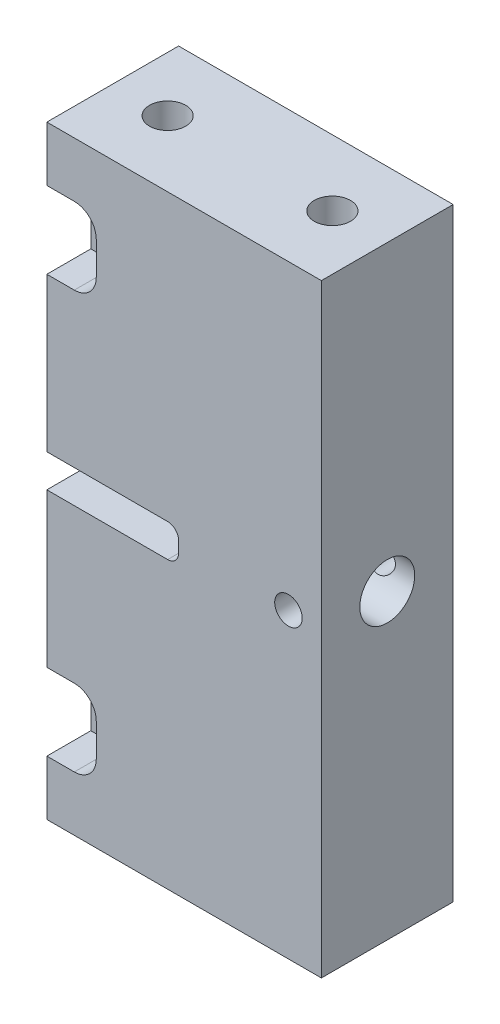
SolidWorks part; units mm, degrees
material "6061铝"
ref_plane "前视基准面" through (0, 0, 0) normal (0, 0, 1) x (1, 0, 0)
ref_plane "上视基准面" through (0, 0, 0) normal (0, 1, 0) x (1, 0, 0)
ref_plane "右视基准面" through (0, 0, 0) normal (1, 0, 0) x (0, 0, -1)
sketch "草图1" plane through (0, 0, 0) normal (1, 0, 0) x (0, 0, -1)
  line L1 (-6, 27.5) -> (6, 27.5)
  line L2 (-6, 27.5) -> (-6, -27.5)
  line L3 (-6, -27.5) -> (6, -27.5)
  line L4 (6, 27.5) -> (6, -27.5)
  line L5 (-6, 27.5) -> (6, -27.5) construction
  line L6 (-6, -27.5) -> (6, 27.5) construction
  point P0 (0, 0)
  dimension "D1" = 12
  dimension "D2" = 55
extrude "凸台-拉伸1" add sketch "草图1" along normal blind 25
sketch "草图2" plane through (25, 0, 0) normal (1, 0, 0) x (0, 0, -1)
  circle A0 centre (0, 0) radius 1.1
  dimension "D1" = 2.2
extrude "切除-拉伸1" cut sketch "草图2" against normal blind 25
sketch "草图3" plane through (25, 0, 0) normal (1, 0, 0) x (0, 0, -1)
  circle A0 centre (0, 0) radius 2.5
  dimension "D1" = 5
extrude "切除-拉伸2" cut sketch "草图3" against normal blind 8
chamfer "倒角1" [suppressed] distance 1 angle 45
sketch "草图4" plane through (0, 0, 6) normal (0, 0, 1) x (1, 0, 0)
  line L0 (0, 27.5) -> (0, -27.5) construction
  line L1 (-12, 1.5) -> (12, 1.5)
  line L2 (-12, 1.5) -> (-12, -1.5)
  line L3 (-12, -1.5) -> (12, -1.5)
  line L4 (12, 1.5) -> (12, -1.5)
  line L5 (-12, 1.5) -> (12, -1.5) construction
  line L6 (-12, -1.5) -> (12, 1.5) construction
  point P0 (0, 0)
  dimension "D1" = 12
  dimension "D2" = 3
extrude "切除-拉伸3" cut sketch "草图4" against normal blind 6
hole_wizard "M4 螺纹孔1" positions "草图6" profile "草图7" tap size "M4" standard "GB"
sketch "草图6" plane through (0, 27.5, 0) normal (0, 1, 0) x (1, 0, 0)
  line L3 (12.5, 6) -> (12.5, -10.1356) construction
  line L4 (25, 6) -> (0, 6) construction
  point P0 (5, 0)
  point P14 (20, 0)
  dimension "D1" = 15
sketch "草图7" plane through (5, 27.5, 0) normal (1, 0, 0) x (0, 0, 1)
  line L0 (0, 0) -> (0, 11.0914)
  line L1 (0, 11.0914) -> (1.65, 10.1)
  line L2 (1.65, 10.1) -> (1.65, 0)
  line L5 (1.65, 0) -> (0, 0)
  line L10 (0, 11.0914) -> (-1.65, 10.1) construction
  line L11 (0, -6.35) -> (0, 107.95) construction
  dimension "螺纹孔钻头直径" = 3.3
  dimension "螺纹孔钻头深度" = 10.1
  dimension "导头角度" = 118
cosmetic thread "孔螺蚊线1" parameters "D1"=8, "D2"=4
cosmetic thread "孔螺蚊线2" parameters "D1"=8, "D2"=4
mirror "镜向1" about plane through (0, 0, 0) normal (0, 1, 0) of "M4 螺纹孔1"
fillet "圆角1" radius 1 2 edges at (12, -1.5, 3) (12, 1.5, 3)
sketch "草图9" plane through (0, 0, 6) normal (0, 0, 1) x (1, 0, 0)
  line L1 (0, 27.5) -> (0, 1.5) construction
  line L2 (-4.5, 22.5) -> (2.5, 22.5)
  line L3 (-4.5, 22.5) -> (-4.5, 15.5)
  line L4 (-4.5, 15.5) -> (2.5, 15.5)
  line L5 (4.5, 20.5) -> (4.5, 17.5)
  line L6 (-4.5, 22.5) -> (4.5, 15.5) construction
  line L7 (0, 0) -> (40.0429, 0) construction
  line L8 (-4.5, 15.5) -> (4.5, 22.5) construction
  arc A0 (4.5, 17.5) -> (2.5, 15.5) centre (2.5, 17.5) cw
  arc A1 (4.5, 20.5) -> (2.5, 22.5) centre (2.5, 20.5) ccw
  point P0 (0, 19)
  dimension "D1" = 19
  dimension "D2" = 2
  dimension "D3" = 4.5
  dimension "D4" = 7
extrude "切除-拉伸4" cut sketch "草图9" against normal blind 4
mirror "镜向2" about plane through (0, 0, 0) normal (0, 1, 0) of "切除-拉伸4"
hole_wizard "M3 螺纹孔1" positions "草图10" profile "草图11" tap size "M3" standard "GB" end condition through all
sketch "草图10" plane through (0, 0, 6) normal (0, 0, 1) x (1, 0, 0)
  line L0 (25, 27.5) -> (25, -27.5) construction
  point P0 (22, 0)
  dimension "D1" = 3
sketch "草图11" plane through (22, 0, 6) normal (1, 0, 0) x (0, -1, 0)
  line L0 (0, 0) -> (0, 12)
  line L1 (0, 12) -> (1.25, 12)
  line L2 (1.25, 12) -> (1.25, 0)
  line L5 (1.25, 0) -> (0, 0)
  line L11 (0, -6.35) -> (0, 107.95) construction
  dimension "通孔螺纹孔钻头直径" = 2.5
  dimension "通孔螺纹孔钻头深度" = 12
cosmetic thread "孔螺蚊线3" parameters "D2"=3
chamfer "倒角2" [suppressed] distance 0.5 angle 45
fillet "圆角2" radius 1 1 edges at (17, 0, -1.1)
